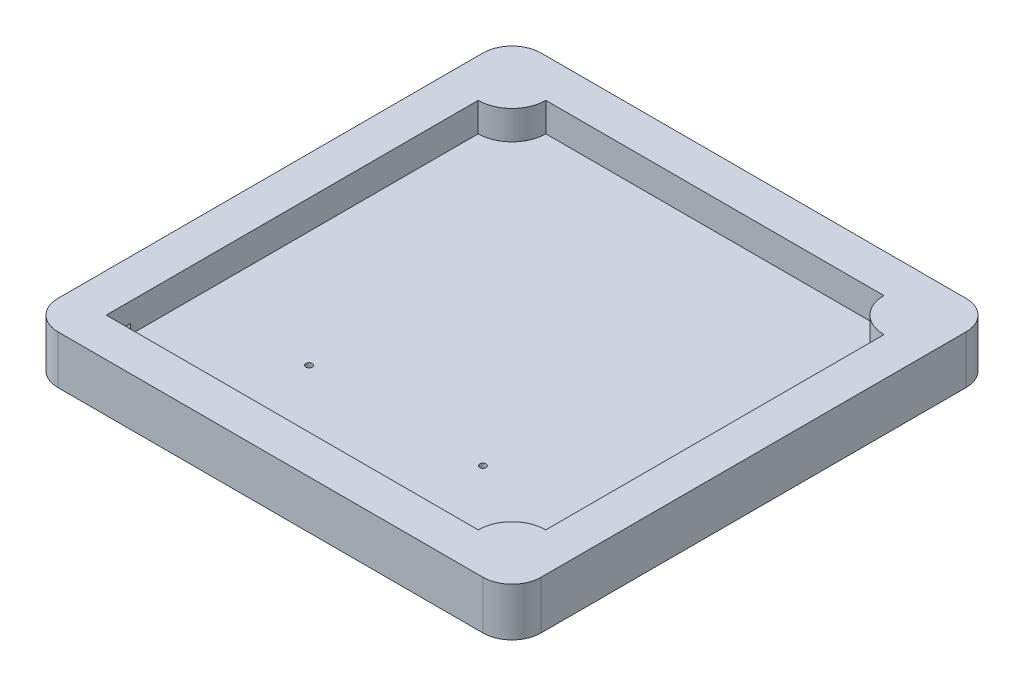
SolidWorks part; units mm, degrees
ref_plane "Front Plane" through (0, 0, 0) normal (0, 0, 1) x (1, 0, 0)
ref_plane "Top Plane" through (0, 0, 0) normal (0, 1, 0) x (1, 0, 0)
ref_plane "Right Plane" through (0, 0, 0) normal (1, 0, 0) x (0, 0, -1)
sketch "Sketch1" plane through (0, 0, 0) normal (0, 1, 0) x (1, 0, 0)
  line L1 (-220, -250) -> (220, -250)
  line L2 (-250, -220) -> (-250, 220)
  line L3 (-220, 250) -> (220, 250)
  line L4 (250, -220) -> (250, 220)
  line L5 (-250, -250) -> (250, 250) construction
  line L6 (-250, 250) -> (250, -250) construction
  arc A0 (-220, -250) -> (-250, -220) centre (-220, -220) cw
  arc A1 (-250, 220) -> (-220, 250) centre (-220, 220) cw
  arc A2 (250, 220) -> (220, 250) centre (220, 220) ccw
  arc A3 (220, -250) -> (250, -220) centre (220, -220) ccw
  point P0 (0, 0)
  dimension "D1" = 30
  dimension "D2" = 30
  dimension "D3" = 30
  dimension "D4" = 30
  dimension "D5" = 500
  dimension "D6" = 500
extrude "Boss-Extrude1" add sketch "Sketch1" along normal blind 50
sketch "Sketch2" plane through (0, 50, 0) normal (0, 1, 0) x (1, 0, 0)
  line L0 (-404.0969, 0) -> (455.3011, 0) construction
  line L5 (0, 372.5472) -> (0, -382.5149) construction
  line L7 (-175, -210) -> (175, -210)
  line L8 (-210, -175) -> (-210, 175)
  line L9 (-175, 210) -> (175, 210)
  line L10 (210, -175) -> (210, 175)
  line L11 (-210, -210) -> (210, 210) construction
  line L12 (-210, 210) -> (210, -210) construction
  arc A1 (175, 210) -> (210, 175) centre (210, 210) ccw
  arc A3 (-175, 210) -> (-210, 175) centre (-210, 210) cw
  arc A8 (-175, -210) -> (-210, -175) centre (-210, -210) ccw
  arc A9 (175, -210) -> (210, -175) centre (210, -210) cw
  point P4 (0, 0)
  dimension "D1" = 420
  dimension "D2" = 420
extrude "Cut-Extrude1" cut sketch "Sketch2" against normal blind 30
sketch "Sketch3" plane through (0, 0, 0) normal (0, -1, 0) x (1, 0, 0)
  line L0 (-408.9721, 0) -> (462.7606, 0) construction
  line L1 (0, 284.5182) -> (0, -260.0804) construction
  circle A0 centre (-210, 210) radius 25
  circle A1 centre (210, 210) radius 25
  circle A2 centre (210, -210) radius 25
  circle A3 centre (-210, -210) radius 25
  dimension "D1" = 210
  dimension "D2" = 210
extrude "Cut-Extrude2" cut sketch "Sketch3" against normal blind 30
sketch "Sketch8" plane through (0, 0, 0) normal (0, 1, 0) x (1, 0, 0)
  line L0 (0, 250) -> (0, -250) construction
  line L1 (220, 250) -> (-220, 250) construction
  line L2 (-220, -250) -> (220, -250) construction
  line L3 (-175, -210) -> (175, -210) construction
  line L4 (-175, -210) -> (175, -210) construction
  point P8 (-90, -200)
  point P12 (90, -120)
  point P14 (-90, -120)
  point P38 (90, -200)
  dimension "D1" = 10
  dimension "D2" = 90
  dimension "D3" = 10
  dimension "D4" = 90
  dimension "D5" = 180
  dimension "D6" = 90
  dimension "D7" = 80
  dimension "D8" = 80
hole_wizard "CBORE for M6 Hexagon head bolts-Full thread-grade C1" positions "Sketch8" profile "Sketch9" counterbore size "M6" standard "GB" end condition through all
sketch "Sketch9" plane through (90, 0, 200) normal (1, 0, 0) x (0, 0, -1)
  line L0 (0, 0) -> (0, 50)
  line L1 (0, 50) -> (3.3, 50)
  line L3 (3.3, 50) -> (3.3, 0.5)
  line L4 (3.3, 0.5) -> (6.5, 0.5)
  line L5 (6.5, 0.5) -> (6.5, 0)
  line L7 (6.5, 0) -> (0, 0)
  line L11 (0, -6.35) -> (0, 107.95) construction
  dimension "通孔孔直径" = 6.6
  dimension "通孔孔深度" = 50
  dimension "柱形沉头孔直径" = 13
  dimension "柱形沉头孔深度" = 0.5
sketch "Sketch10" plane through (0, 50, 0) normal (0, 1, 0) x (1, 0, 0)
  line L0 (-210, -175) -> (-210, -210)
  line L1 (-175, -210) -> (-210, -210)
  arc A0 (-210, -175) -> (-175, -210) centre (-210, -210) cw
extrude "Cut-Extrude8" cut sketch "Sketch10" against normal blind 30
